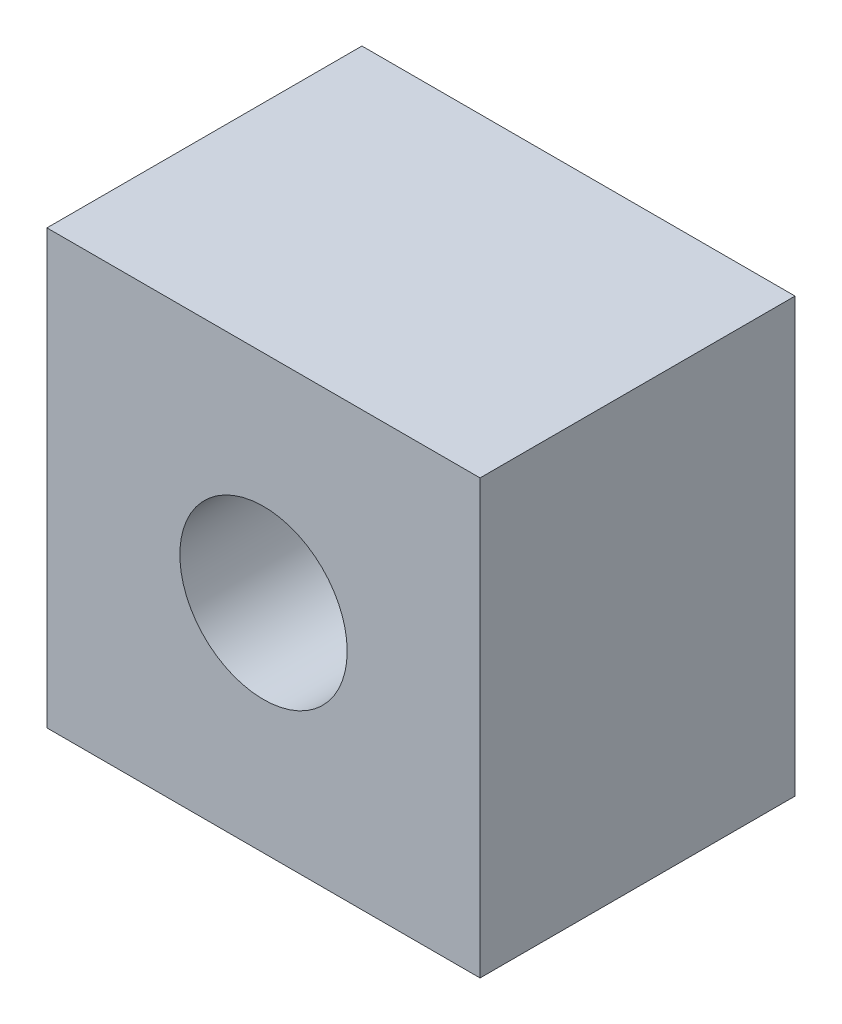
from build123d import *

# Parameters (mm, degrees)
SKETCH1_W              = 22
SKETCH1_H              = 22
BOSS_EXTRUDE1_DEPTH    = 16
M10_TAPPED_HOLE1_D     = 8.5
M10_TAPPED_HOLE1_DEPTH = 27.5
M10_TAPPED_HOLE1_TIP   = 2.553657631


with BuildPart() as part:
    # Sketch1 → Boss-Extrude1 (new body)
    with BuildSketch(Plane.XY):
        Rectangle(SKETCH1_W, SKETCH1_H)
    extrude(amount=BOSS_EXTRUDE1_DEPTH)

    # M10 Tapped Hole1
    with Locations(Plane.XY.offset(16)):
        with Locations((0, 0)):
            Hole(M10_TAPPED_HOLE1_D / 2, depth=M10_TAPPED_HOLE1_DEPTH)
            with Locations((0, 0, -(M10_TAPPED_HOLE1_DEPTH + M10_TAPPED_HOLE1_TIP / 2))):  # 118° drill point
                Cone(0, M10_TAPPED_HOLE1_D / 2, M10_TAPPED_HOLE1_TIP, mode=Mode.SUBTRACT)


solid = part.part
